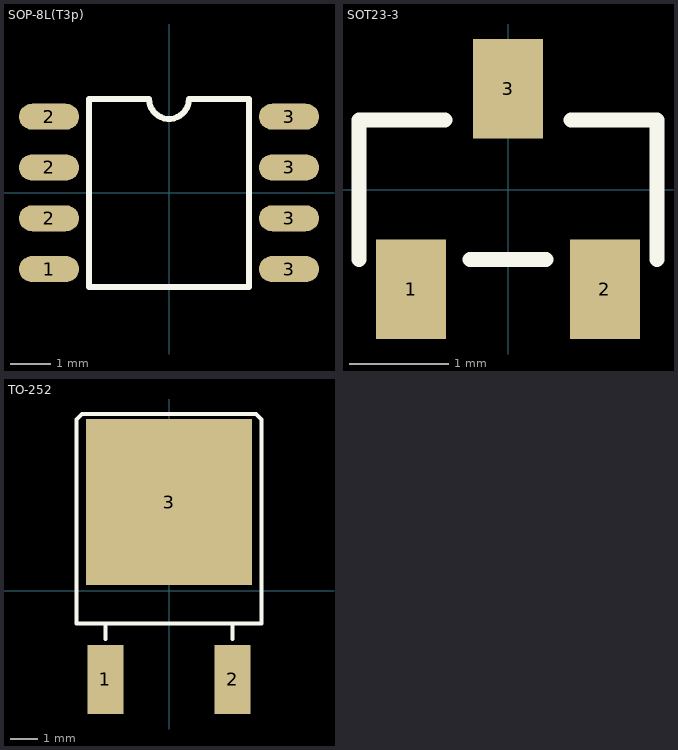
[diagram p0: the footprints below, top view; thin cyan lines are the x and y axes]
# Altium footprint library MISC75736.PcbLib: 19 footprints (part 2 of 2)
Each footprint in its own frame and in the unit in brackets; x right, y up, seen from the top. Pads: shape width x height; smd on the part's side, far side on the other; paste and mask are expansions set on the pad; w line width, h text height; cw(c..) or ccw(c..) is an arc to the next point about the centre after c.

## SOP-8L(T3p) [mm] "chip MOS (non-standard)"
height 0.5
pads (8):
  oval 1.5x0.65 smd: 1(-3,-1.905) 2(-3,-0.635) 2(-3,0.635) 2(-3,1.905) 3(3,-1.905) 3(3,-0.635) 3(3,0.635) 3(3,1.905)
Top Overlay:
  lines w0.15: -2,-2.35 -2,2.35 -0.5,2.35 ccw(c0,2.35) 0.5,2.35 2,2.35 2,-2.35 -2,-2.35

## SOT23-3 [mm] "chip IC/MOS*"
pads (3):
  rect 0.7x1 smd: 1(-0.975,-1) 2(0.975,-1) 3(0,1.016)
Top Overlay:
  lines w0.15: -1.5,-0.7 -1.5,0.7 -0.635,0.7 ; -0.381,-0.7 0.381,-0.7 ; 0.635,0.7 1.5,0.7 1.5,-0.7

## TO-252 [mm]
height 1.75
pads (3):
  rect 1.3x2.5 smd: 1(-2.3,-3.212) 2(2.3,-3.212)
  rect 6x6 smd: 3(0,3.213)
Top Overlay:
  lines w0.15: -2.3,-1.75 -2.3,-1.18 ; 2.3,-1.75 2.3,-1.18 ; -3.35,-1.18 3.35,-1.18 3.35,6.19 3.35,6.2 3.15,6.4 -3.15,6.4 -3.35,6.2 -3.35,-1.18